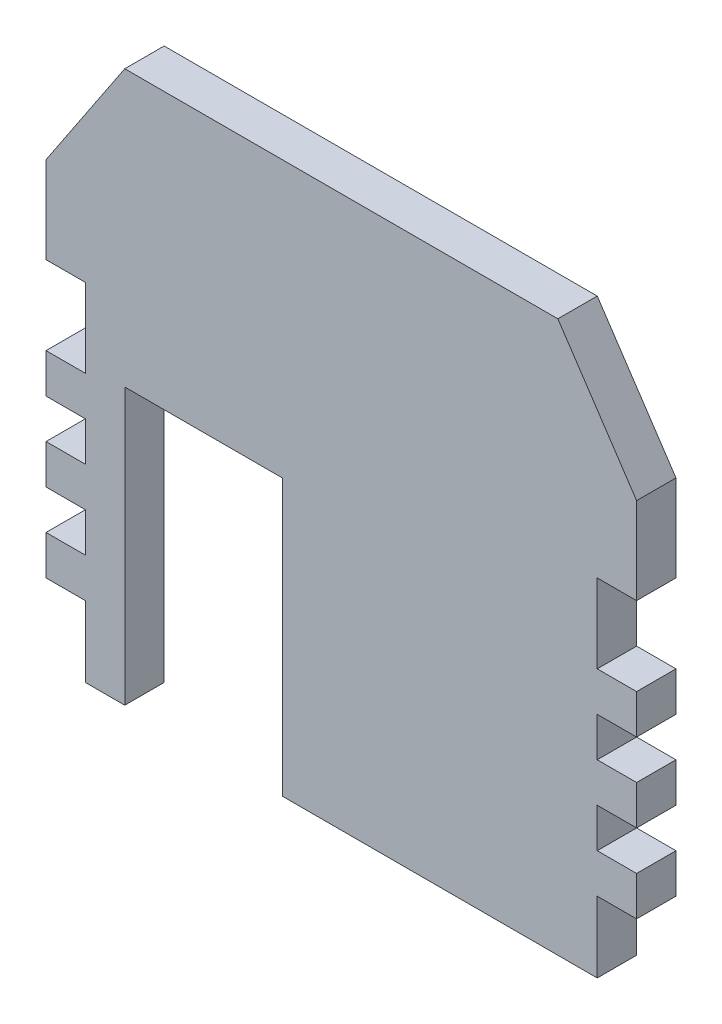
SolidWorks part; units mm, degrees
ref_plane "Front Plane" through (0, 0, 0) normal (0, 0, 1) x (1, 0, 0)
ref_plane "Top Plane" through (0, 0, 0) normal (0, 1, 0) x (1, 0, 0)
ref_plane "Right Plane" through (0, 0, 0) normal (1, 0, 0) x (0, 0, -1)
other "Configuration Table"
sketch "Sketch1" plane through (0, 0, 0) normal (0, 0, 1) x (1, 0, 0)
  line L1 (37.5, -37.5) -> (-37.5, -37.5)
  line L2 (37.5, -37.5) -> (37.5, 37.5)
  line L3 (37.5, 37.5) -> (-37.5, 37.5)
  line L4 (-37.5, -37.5) -> (-37.5, 37.5)
  line L5 (37.5, -37.5) -> (-37.5, 37.5) construction
  line L6 (37.5, 37.5) -> (-37.5, -37.5) construction
  point P0 (0, 0)
  dimension "D1" = 75
  dimension "D2" = 75
extrude "Boss-Extrude1" add sketch "Sketch1" along normal blind 5
sketch "Sketch2" plane through (0, 0, 5) normal (0, 0, 1) x (1, 0, 0)
  line L0 (-27.5, 37.5) -> (-37.5, 22.5)
  line L1 (37.5, 37.5) -> (-37.5, 37.5) construction
  line L2 (-37.5, 37.5) -> (-37.5, -37.5) construction
  line L3 (-37.5, 22.5) -> (-37.5, 37.5)
  line L4 (-37.5, 37.5) -> (-27.5, 37.5)
  line L5 (37.5, 37.5) -> (27.5, 37.5)
  line L6 (27.5, 37.5) -> (37.5, 22.5)
  line L7 (37.5, -37.5) -> (37.5, 37.5) construction
  line L8 (37.5, 22.5) -> (37.5, 37.5)
  dimension "D1" = 10
  dimension "D2" = 15
  dimension "D3" = 10
  dimension "D4" = 15
extrude "Cut-Extrude1" cut sketch "Sketch2" against normal blind 5
sketch "Sketch3" plane through (0, 0, 5) normal (0, 0, 1) x (1, 0, 0)
  line L0 (-37.5, -37.5) -> (37.5, -37.5) construction
  line L1 (-27.5, -37.5) -> (-7.5, -37.5)
  line L2 (-27.5, -37.5) -> (-27.5, 2.5)
  line L3 (-27.5, 2.5) -> (-7.5, 2.5)
  line L4 (-7.5, -37.5) -> (-7.5, 2.5)
  line L5 (-37.5, 22.5) -> (-37.5, -37.5) construction
  dimension "D1" = 10
  dimension "D2" = 40
  dimension "D3" = 20
extrude "Cut-Extrude2" cut sketch "Sketch3" against normal blind 5
sketch "Sketch4" plane through (0, 0, 5) normal (0, 0, 1) x (1, 0, 0)
  line L0 (-37.5, 22.5) -> (-37.5, -37.5) construction
  line L1 (-37.5, -37.5) -> (-32.5, -37.5)
  line L2 (-37.5, -37.5) -> (-37.5, -23.5)
  line L3 (-37.5, -23.5) -> (-32.5, -23.5)
  line L4 (-32.5, -37.5) -> (-32.5, -23.5)
  line L6 (-37.5, -18.5) -> (-32.5, -18.5)
  line L7 (-37.5, -18.5) -> (-37.5, -13.5)
  line L8 (-37.5, -13.5) -> (-32.5, -13.5)
  line L9 (-32.5, -18.5) -> (-32.5, -13.5)
  line L14 (-37.5, -37.5) -> (-27.5, -37.5) construction
  line L19 (-37.5, -8.5) -> (-32.5, -8.5)
  line L20 (-37.5, -8.5) -> (-37.5, -3.5)
  line L21 (-37.5, -3.5) -> (-32.5, -3.5)
  line L22 (-32.5, -8.5) -> (-32.5, -3.5)
  line L24 (-37.5, 1.5) -> (-32.5, 1.5)
  line L25 (-37.5, 1.5) -> (-37.5, 11.5)
  line L26 (-37.5, 11.5) -> (-32.5, 11.5)
  line L27 (-32.5, 1.5) -> (-32.5, 11.5)
  dimension "D1" = 14
  dimension "D2" = 5
  dimension "D3" = 5
  dimension "D4" = 5
  dimension "D5" = 5
  dimension "D6" = 5
  dimension "D7" = 14
  dimension "D8" = 5
  dimension "D9" = 5
  dimension "D10" = 5
  dimension "D11" = 10
  dimension "D12" = 5
extrude "Cut-Extrude3" cut sketch "Sketch4" against normal up to next
sketch "Sketch5" plane through (0, 0, 5) normal (0, 0, 1) x (1, 0, 0)
  line L19 (37.5, -37.5) -> (37.5, 22.5) construction
  line L20 (37.5, -18.5) -> (32.5, -18.5)
  line L21 (37.5, -18.5) -> (37.5, -13.5)
  line L22 (37.5, -13.5) -> (32.5, -13.5)
  line L23 (32.5, -18.5) -> (32.5, -13.5)
  line L25 (37.5, -8.5) -> (32.5, -8.5)
  line L26 (37.5, -8.5) -> (37.5, -3.5)
  line L27 (37.5, -3.5) -> (32.5, -3.5)
  line L28 (32.5, -8.5) -> (32.5, -3.5)
  line L33 (37.5, -37.5) -> (32.5, -37.5)
  line L34 (37.5, -37.5) -> (37.5, -23.5)
  line L35 (37.5, -23.5) -> (32.5, -23.5)
  line L36 (32.5, -37.5) -> (32.5, -23.5)
  line L38 (37.5, 1.5) -> (32.5, 1.5)
  line L39 (37.5, 1.5) -> (37.5, 11.5)
  line L40 (37.5, 11.5) -> (32.5, 11.5)
  line L41 (32.5, 1.5) -> (32.5, 11.5)
  point P18 (35, 1.5)
  dimension "D1" = 14
  dimension "D2" = 5
  dimension "D3" = 5
  dimension "D4" = 19
  dimension "D5" = 5
  dimension "D6" = 5
  dimension "D7" = 5
  dimension "D8" = 5
  dimension "D9" = 5
  dimension "D10" = 10
  dimension "D11" = 5
extrude "Cut-Extrude4" cut sketch "Sketch5" against normal up to next
sketch "Sketch7" plane through (0, 0, 5) normal (0, 0, 1) x (1, 0, 0)
  line L0 (32.5, -23.5) -> (32.5, -37.5) construction
  line L1 (-32.5, -37.5) -> (32.5, -37.5)
  line L2 (-32.5, -37.5) -> (-32.5, -32.5)
  line L3 (-32.5, -32.5) -> (32.5, -32.5)
  line L4 (32.5, -37.5) -> (32.5, -32.5)
  dimension "D1" = 5
extrude "Cut-Extrude5" cut sketch "Sketch7" against normal blind 10
